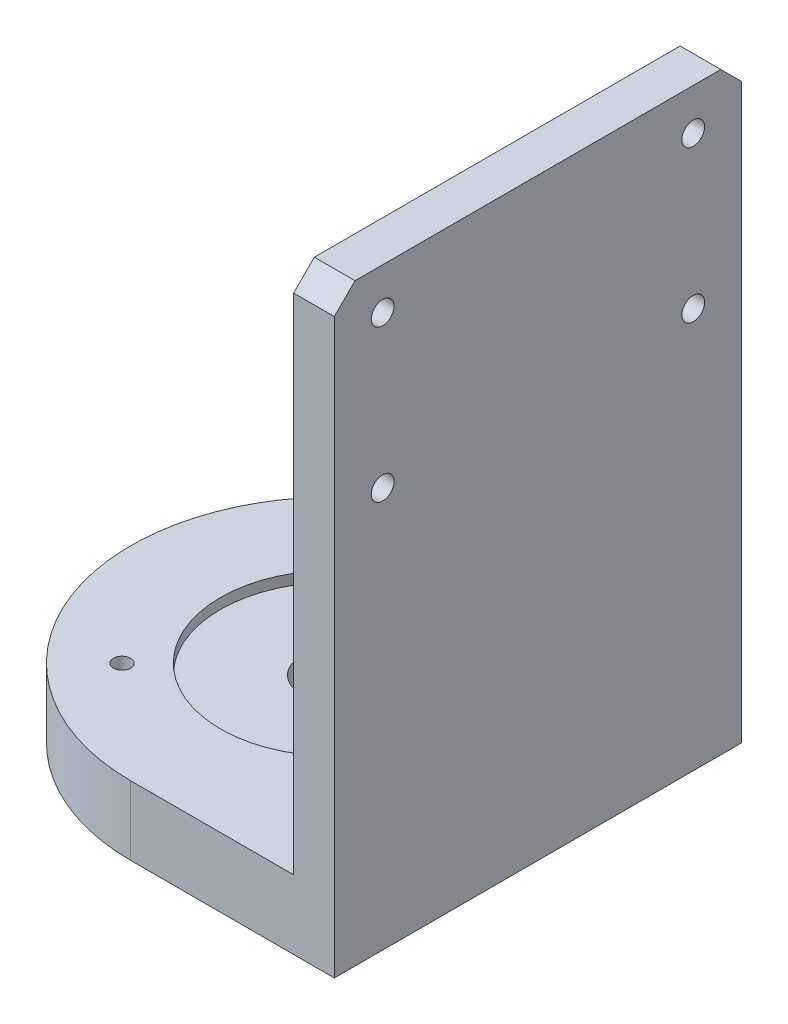
from build123d import *

# Parameters (mm, degrees)
BOSS_EXTRUDE1_DEPTH = 29.5
SKETCH2_R           = 4.8
CUT_EXTRUDE1_DEPTH  = 10
SKETCH4_R           = 16.5
CUT_EXTRUDE2_DEPTH  = 1.5
M3_TAPPED_HOLE1_D   = 2.5
CHAMFER1_SIZE       = 3
M4_TAPPED_HOLE1_D   = 3.3


with BuildPart() as part:
    # Sketch1 → Boss-Extrude1 (new, symmetric)
    with BuildSketch(Plane.XY):
        Polygon((15.9, 0.233022363), (-43.1, 0.233022363), (-43.1, 10.233022363), (10, 10.233022363), (10, 86.233022363), (15.9, 86.233022363), align=None)
    extrude(amount=BOSS_EXTRUDE1_DEPTH, both=True)

    # Sketch2 → Cut-Extrude1 (cut)
    with BuildSketch(Plane.XZ.offset(-0.233022363)):
        with BuildLine():
            ThreePointArc((-43.1, 0), (-34.459650045, 20.859650045), (-13.6, 29.5))
            Line((-13.6, 29.5), (-43.1, 29.5))
            Line((-43.1, 29.5), (-43.1, 0))
        make_face()
        with BuildLine():
            ThreePointArc((-13.6, -29.5), (-34.459650045, -20.859650045), (-43.1, 0))
            Line((-43.1, 0), (-43.1, -29.5))
            Line((-43.1, -29.5), (-13.6, -29.5))
        make_face()
        with Locations((-13.6, 0)):
            Circle(SKETCH2_R)
    extrude(amount=-CUT_EXTRUDE1_DEPTH, mode=Mode.SUBTRACT)

    # Sketch4 → Cut-Extrude2 (cut)
    with BuildSketch(Plane(origin=(0, 10.233022363, 0), x_dir=(1, 0, 0), z_dir=(0, 1, 0))):
        with Locations(Location((-13.6, 0, 0), (0, 0, 180))):
            Circle(SKETCH4_R)
    extrude(amount=-CUT_EXTRUDE2_DEPTH, mode=Mode.SUBTRACT)

    # M3 Tapped Hole1 (through all)
    with Locations(Plane(origin=(0, 10.233022363, 0), x_dir=(1, 0, 0), z_dir=(0, 1, 0))):
        with Locations((-28.979572491, -15.379572491), (-28.979572491, 15.379572491), (1.779572491, 15.379572491), (1.779572491, -15.379572491)):
            Hole(M3_TAPPED_HOLE1_D / 2)

    # Chamfer1
    chamfer1_edges = [part.edges().sort_by_distance(p)[0] for p in [
        (12.95, 86.233022363, 29.5),
        (12.95, 86.233022363, -29.5),
    ]]
    chamfer(chamfer1_edges, length=CHAMFER1_SIZE)

    # M4 Tapped Hole1 (through all)
    with Locations(Plane.ZY.offset(-10)):
        with Locations((-22.5, 80.233022363), (-22.5, 58.233022363), (22.5, 58.233022363), (22.5, 80.233022363)):
            Hole(M4_TAPPED_HOLE1_D / 2)


solid = part.part
